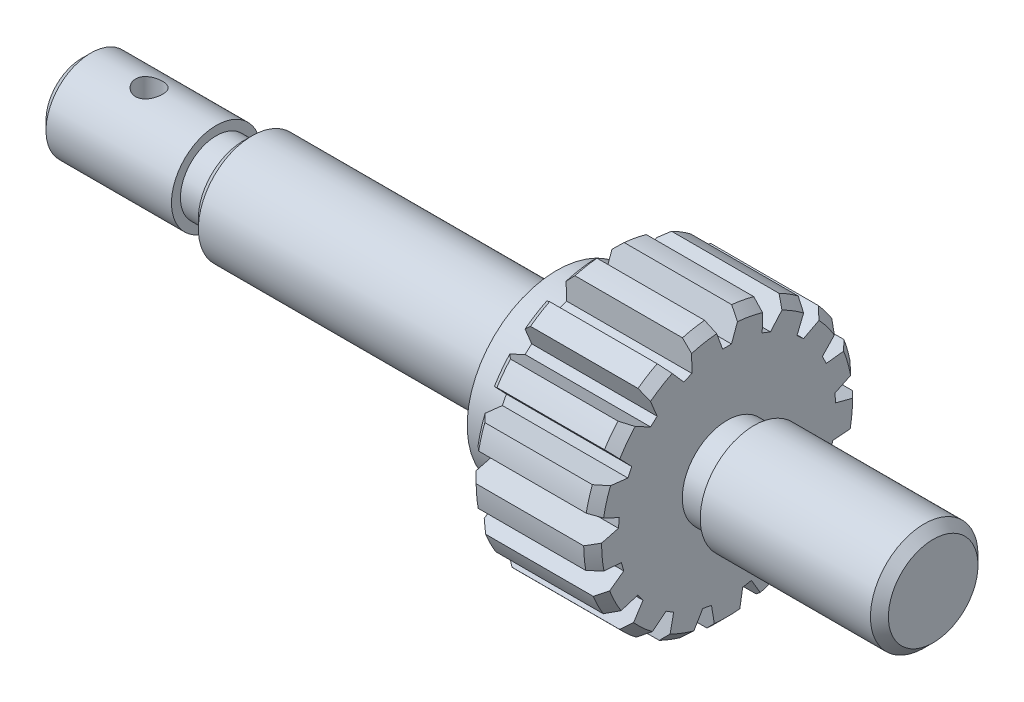
SolidWorks part; units mm, degrees
ref_plane "Front Plane" through (0, 0, 0) normal (0, 0, 1) x (1, 0, 0)
ref_plane "Top Plane" through (0, 0, 0) normal (0, 1, 0) x (1, 0, 0)
ref_plane "Right Plane" through (0, 0, 0) normal (1, 0, 0) x (0, 0, -1)
other "Configuration Table"
sketch "Sketch1" plane through (0, 0, 0) normal (1, 0, 0) x (0, 0, -1)
  circle A0 centre (0, 0) radius 5
  dimension "D1" = 10
extrude "Boss-Extrude1" add sketch "Sketch1" along normal blind 15
sketch "Sketch2" plane through (15, 0, 0) normal (1, 0, 0) x (0, 0, -1)
  circle A0 centre (0, 0) radius 4
  dimension "D1" = 8
extrude "Boss-Extrude2" add sketch "Sketch2" along normal blind 3
sketch "Sketch3" plane through (18, 0, 0) normal (1, 0, 0) x (0, 0, -1)
  circle A0 centre (0, 0) radius 6
  dimension "D1" = 12
extrude "Boss-Extrude3" add sketch "Sketch3" along normal blind 35
sketch "Sketch4" plane through (53, 0, 0) normal (1, 0, 0) x (0, 0, -1)
  circle A0 centre (0, 0) radius 10
  dimension "D1" = 20
extrude "Boss-Extrude4" add sketch "Sketch4" along normal blind 5
sketch "Sketch5" plane through (58, 0, 0) normal (1, 0, 0) x (0, 0, -1)
  circle A0 centre (0, 0) radius 15
  dimension "D1" = 30
extrude "Boss-Extrude5" add sketch "Sketch5" along normal blind 14
sketch "Sketch6" plane through (72, 0, 0) normal (1, 0, 0) x (0, 0, -1)
  circle A0 centre (0, 0) radius 5
  dimension "D1" = 10
extrude "Boss-Extrude6" add sketch "Sketch6" along normal blind 3
sketch "Sketch7" plane through (75, 0, 0) normal (1, 0, 0) x (0, 0, -1)
  circle A0 centre (0, 0) radius 6
  dimension "D1" = 12
extrude "Boss-Extrude7" add sketch "Sketch7" along normal blind 20
chamfer "Chamfer1" distance 1 angle 45 5 edges at (95, 0, -6) (58, 0, -15) (72, 0, -15) (0, 0, -5) (18, 0, -6)
sketch "Sketch8" plane through (58, 0, 0) normal (-1, 0, 0) x (0, 0, 1)
  line L0 (0, 0) -> (0, 22.988) construction
  line L1 (2.1756, 16.7422) -> (-2.1756, 16.7422)
  line L2 (-2.1756, 16.7422) -> (-0.4951, 12.125)
  line L3 (-0.4951, 12.125) -> (0.4951, 12.125)
  line L4 (-1.1775, 14) -> (1.1775, 14) construction
  line L5 (2.1756, 16.7422) -> (0.4951, 12.125)
  point P10 (0, 14)
  point P11 (0, 12.125)
  point P12 (0, 16.7422)
  dimension "D1" = 2.355
  dimension "D2" = 1.875
  dimension "D3" = 14
  dimension "D4" = 20
extrude "Cut-Extrude1" cut sketch "Sketch8" against normal through all both and the other way through all
pattern_circular "CirPattern1" count 17 over 360 about axis through (0, 0, 0) along (1, 0, 0) of "Cut-Extrude1"
sketch "Sketch9" plane through (0, 0, 0) normal (0, 0, 1) x (1, 0, 0)
  line L0 (7.5, 10.1728) -> (7.5, -6.529)
  line L1 (0, 4) -> (0, -4) construction
  dimension "D1" = 7.5
sweep "Cut-Sweep1" cut path "Sketch9" circular profile diameter 3 parameters "D3"=3
